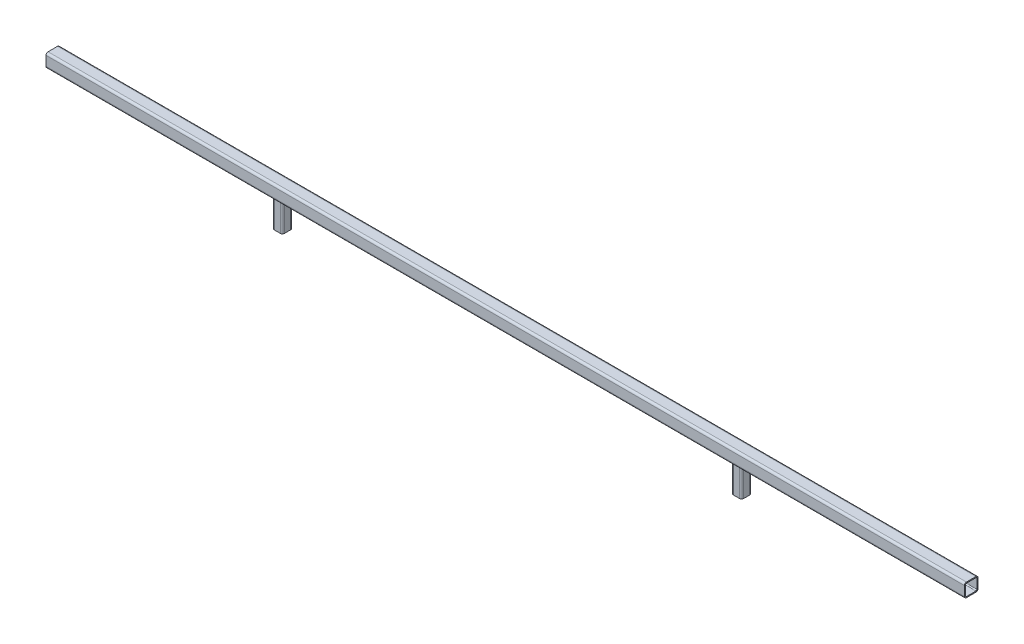
from build123d import *

# Parameters (mm, degrees)
GB_T6728_2002_40_X_40_X_3_1_DEPTH   = 2700
GB_T6728_2002_30_X_30_X_3_1_DEPTH   = 100
GB_T6728_2002_30_X_30_X_3_1_2_DEPTH = 100


with BuildPart() as part:
    # Sketch1 → 冷弯空心方管gb∕t6728-2002 40 X 40 X 3(1) (new body)
    with BuildSketch(Plane(origin=(-1350, 0, 0), x_dir=(0, 0, -1), z_dir=(1, 0, 0))):
        with BuildLine():
            Line((-14, -20), (14, -20))
            ThreePointArc((14, -20), (18.242640687, -18.242640687), (20, -14))
            Line((20, -14), (20, 14))
            ThreePointArc((20, 14), (18.242640687, 18.242640687), (14, 20))
            Line((14, 20), (-14, 20))
            ThreePointArc((-14, 20), (-18.242640687, 18.242640687), (-20, 14))
            Line((-20, 14), (-20, -14))
            ThreePointArc((-20, -14), (-18.242640687, -18.242640687), (-14, -20))
        make_face()
        with BuildLine():
            Line((-14, -17), (14, -17))
            ThreePointArc((14, -17), (16.121320344, -16.121320344), (17, -14))
            Line((17, -14), (17, 14))
            ThreePointArc((17, 14), (16.121320344, 16.121320344), (14, 17))
            Line((14, 17), (-14, 17))
            ThreePointArc((-14, 17), (-16.121320344, 16.121320344), (-17, 14))
            Line((-17, 14), (-17, -14))
            ThreePointArc((-17, -14), (-16.121320344, -16.121320344), (-14, -17))
        make_face(mode=Mode.SUBTRACT)
    extrude(amount=GB_T6728_2002_40_X_40_X_3_1_DEPTH)


with BuildPart() as body_2:
    # Sketch11 → 冷弯空心方管gb∕t6728-2002 30 X 30 X 3(1) (new body)
    with BuildSketch(Plane(origin=(-675, 0, 0), x_dir=(1, 0, 0), z_dir=(0, -1, 0))):
        with BuildLine():
            Line((-9, -15), (9, -15))
            ThreePointArc((9, -15), (13.242640687, -13.242640687), (15, -9))
            Line((15, -9), (15, 9))
            ThreePointArc((15, 9), (13.242640687, 13.242640687), (9, 15))
            Line((9, 15), (-9, 15))
            ThreePointArc((-9, 15), (-13.242640687, 13.242640687), (-15, 9))
            Line((-15, 9), (-15, -9))
            ThreePointArc((-15, -9), (-13.242640687, -13.242640687), (-9, -15))
        make_face()
        with BuildLine():
            Line((-9, -12), (9, -12))
            ThreePointArc((9, -12), (11.121320344, -11.121320344), (12, -9))
            Line((12, -9), (12, 9))
            ThreePointArc((12, 9), (11.121320344, 11.121320344), (9, 12))
            Line((9, 12), (-9, 12))
            ThreePointArc((-9, 12), (-11.121320344, 11.121320344), (-12, 9))
            Line((-12, 9), (-12, -9))
            ThreePointArc((-12, -9), (-11.121320344, -11.121320344), (-9, -12))
        make_face(mode=Mode.SUBTRACT)
    extrude(amount=GB_T6728_2002_30_X_30_X_3_1_DEPTH)

    # Weld Trim 1
    split(bisect_by=Plane.XZ.offset(20), keep=Keep.TOP)


with BuildPart() as body_3:
    # Sketch11 on segment 2 (carried to segment 2) → gb_t6728-2002 30 X 30 X 3_1 2 (new body)
    with BuildSketch(Plane(origin=(675, 0, 0), x_dir=(1, 0, 0), z_dir=(0, -1, 0))):
        with BuildLine():
            Line((-9, -15), (9, -15))
            ThreePointArc((9, -15), (13.242640687, -13.242640687), (15, -9))
            Line((15, -9), (15, 9))
            ThreePointArc((15, 9), (13.242640687, 13.242640687), (9, 15))
            Line((9, 15), (-9, 15))
            ThreePointArc((-9, 15), (-13.242640687, 13.242640687), (-15, 9))
            Line((-15, 9), (-15, -9))
            ThreePointArc((-15, -9), (-13.242640687, -13.242640687), (-9, -15))
        make_face()
        with BuildLine():
            Line((-9, -12), (9, -12))
            ThreePointArc((9, -12), (11.121320344, -11.121320344), (12, -9))
            Line((12, -9), (12, 9))
            ThreePointArc((12, 9), (11.121320344, 11.121320344), (9, 12))
            Line((9, 12), (-9, 12))
            ThreePointArc((-9, 12), (-11.121320344, 11.121320344), (-12, 9))
            Line((-12, 9), (-12, -9))
            ThreePointArc((-12, -9), (-11.121320344, -11.121320344), (-9, -12))
        make_face(mode=Mode.SUBTRACT)
    extrude(amount=GB_T6728_2002_30_X_30_X_3_1_2_DEPTH)

    # Weld Trim 1
    split(bisect_by=Plane.XZ.offset(20), keep=Keep.TOP)


solid = Compound([part.part, body_2.part, body_3.part])
